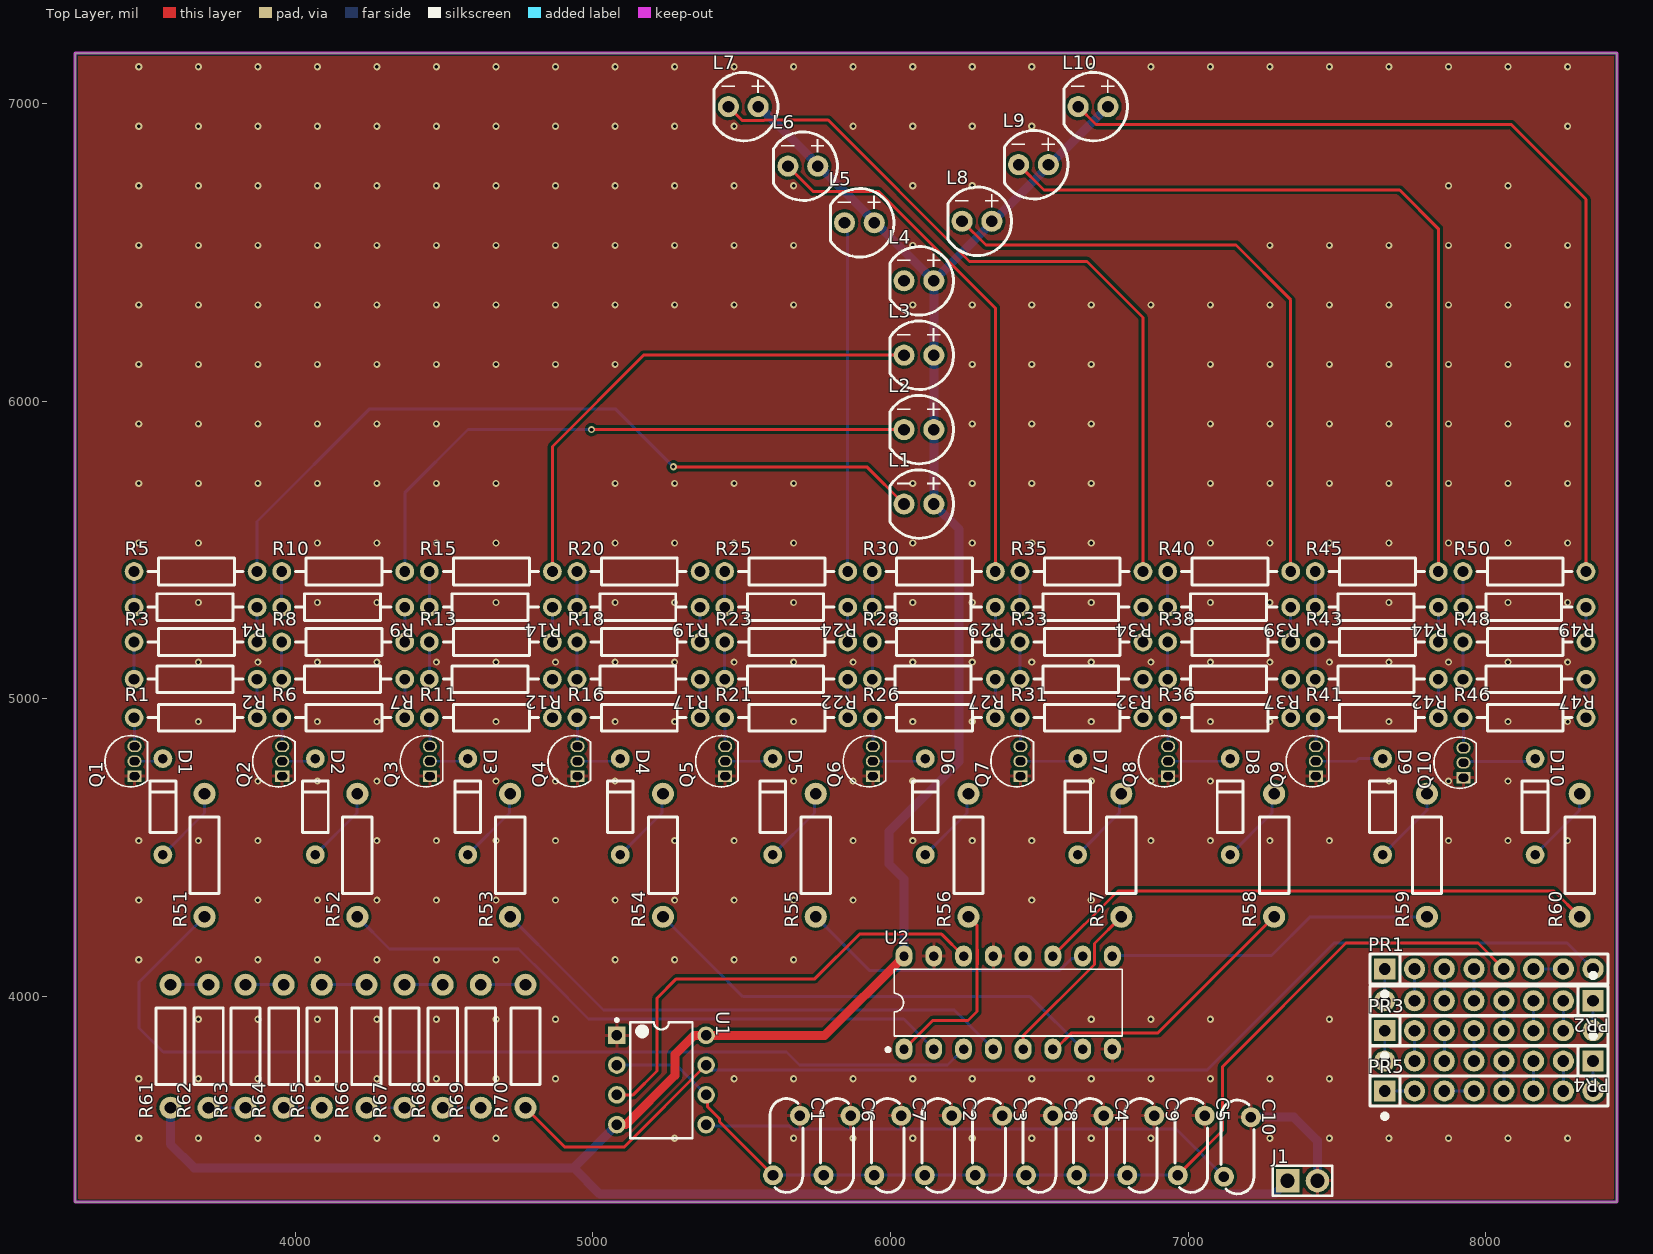
[diagram p0: Top Layer view]
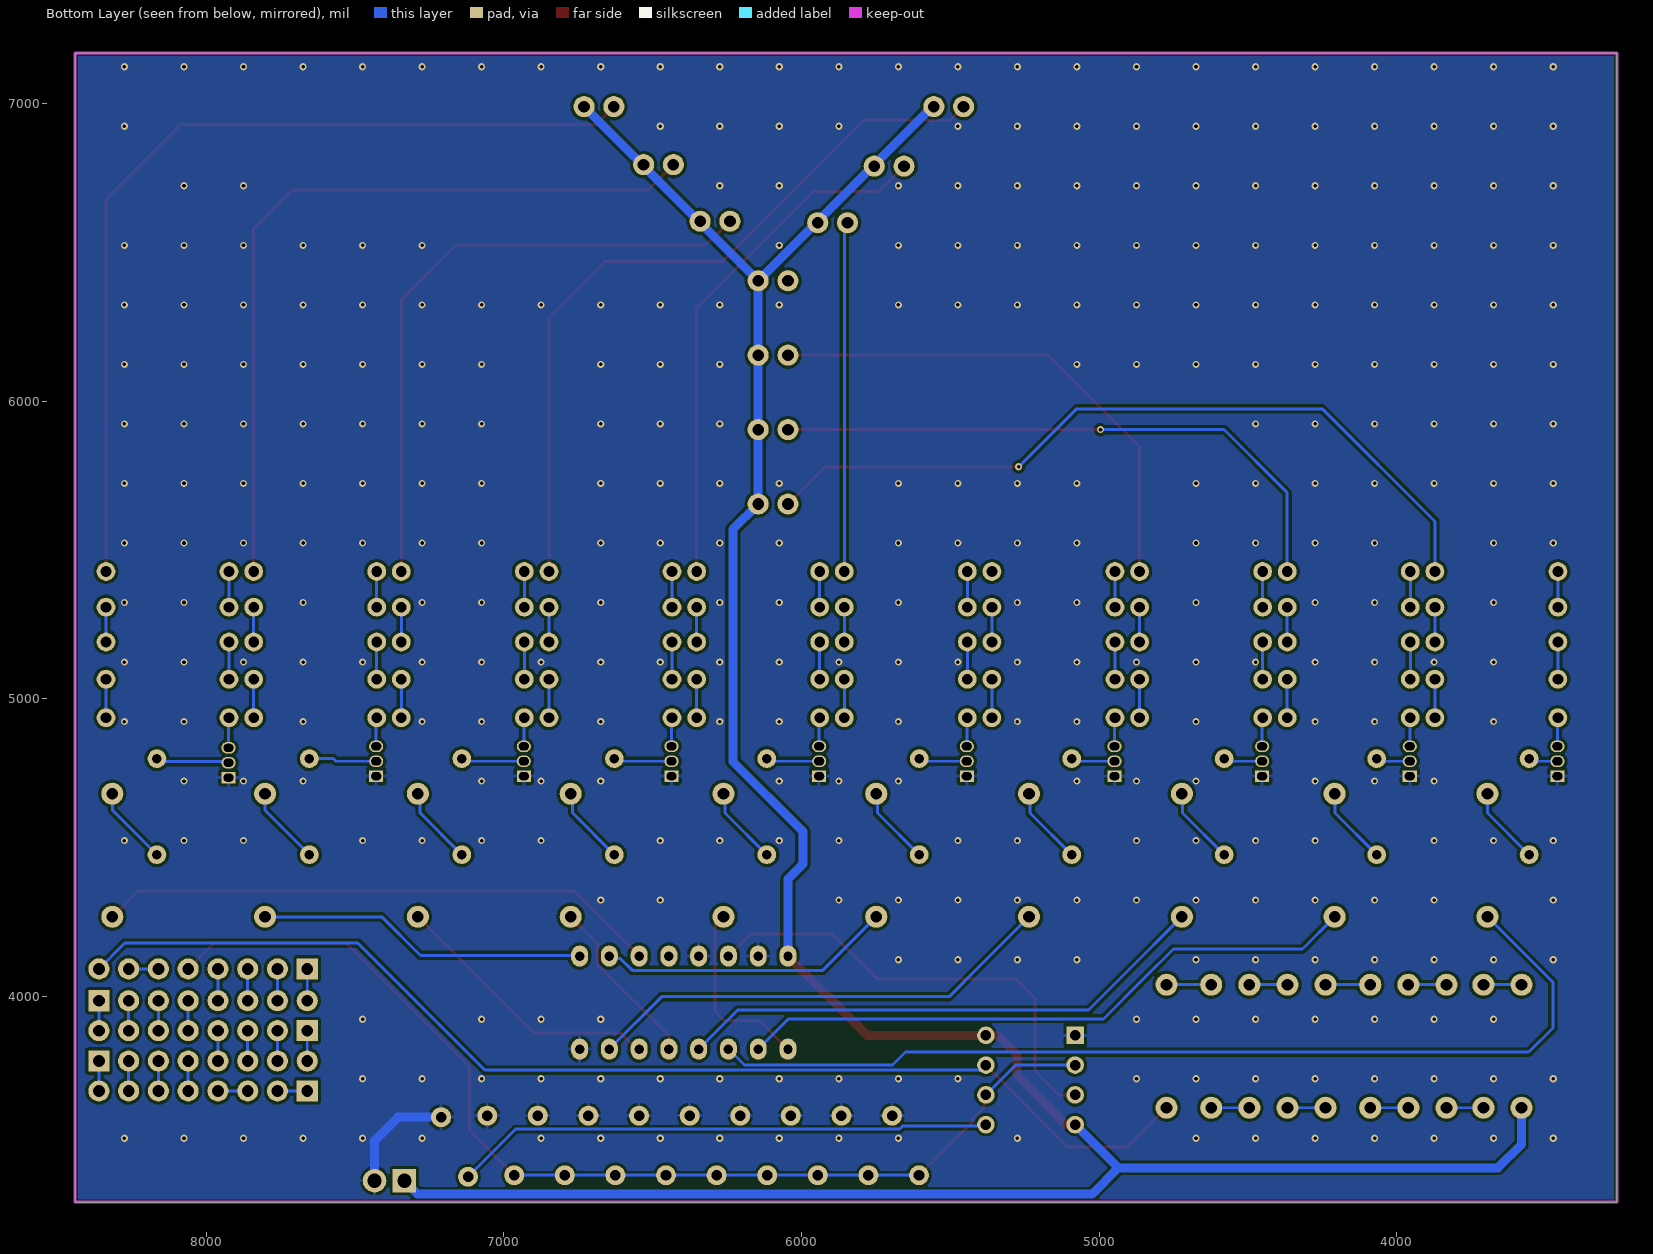
[diagram p1: Bottom Layer view, seen from below]
# Altium PCB MISC51982.pcbdoc
Units mil, origin at the board's own origin, x right, y up, seen from the top; angles counter-clockwise.
Board outline 5180 x 3860 mil, 2 copper layers (Top Layer, Bottom Layer), stack 62.206 mil thick; 118 components, 124 nets, 296 pads, 345 vias.

## Layer stack, top to bottom
Top Solder Mask Layer: solder mask 0.394, Dk 3.3
Top Layer: signal copper 1.379
Dielectric1: surface 59.449, FR4, Dk 4.5
Bottom Layer: signal copper 1.378
Bottom Solder Mask Layer: solder mask 0.394, Dk 3.3

## Board outline
3260,7170 3260,3310 8440,3310 8440,7170

## Design rules (kind name [scope] priority, off if disabled: settings)
BoardOutlineClearance copperThickness2oz_1 [All] p2 off: genericclearance=7.99 ignorepadtopadclearanceinfootprint=FALSE except(0: Arc-SplitContinuation Track-SplitContinuation SMDPad-SplitContinuation THPad-SplitContinuation Via-SplitContinuation Fill-SplitContinuation Region-SplitContinuation Poly-SplitContinuation Text-SplitContinuation Hole-SplitContinuation; 5.98: Arc-CutoutEdge SMDPad-CutoutEdge THPad-CutoutEdge Via-CutoutEdge Fill-CutoutEdge Region-CutoutEdge Text-CutoutEdge; 6.93: Hole-OutlineEdge Hole-CutoutEdge; 10: Poly-OutlineEdge Poly-CutoutEdge; 11.81: Arc-OutlineEdge Track-OutlineEdge SMDPad-OutlineEdge THPad-OutlineEdge Via-OutlineEdge Fill-OutlineEdge Region-OutlineEdge Text-OutlineEdge Track-CutoutEdge)
BoardOutlineClearance Plane_innerPlane_1 [All] p4 off: genericclearance=4.02 ignorepadtopadclearanceinfootprint=FALSE except(0: Arc-SplitContinuation Track-SplitContinuation SMDPad-SplitContinuation THPad-SplitContinuation Via-SplitContinuation Fill-SplitContinuation Region-SplitContinuation Poly-SplitContinuation Text-SplitContinuation Hole-SplitContinuation; 6: SMDPad-CutoutEdge THPad-CutoutEdge Via-CutoutEdge Fill-CutoutEdge Region-CutoutEdge Text-CutoutEdge; 6.93: Hole-OutlineEdge Hole-CutoutEdge; 10: Poly-OutlineEdge Poly-CutoutEdge; 11.8: Arc-OutlineEdge Track-OutlineEdge SMDPad-OutlineEdge THPad-OutlineEdge Via-OutlineEdge Fill-OutlineEdge Region-OutlineEdge Text-OutlineEdge; 11.81: Arc-CutoutEdge Track-CutoutEdge)
BoardOutlineClearance Copper_copperRegion_1 [All] p6 off: genericclearance=4.02 ignorepadtopadclearanceinfootprint=FALSE except(0: Arc-SplitContinuation Track-SplitContinuation SMDPad-SplitContinuation THPad-SplitContinuation Via-SplitContinuation Fill-SplitContinuation Region-SplitContinuation Poly-SplitContinuation Text-SplitContinuation Hole-SplitContinuation; 6: SMDPad-CutoutEdge THPad-CutoutEdge Via-CutoutEdge Fill-CutoutEdge Region-CutoutEdge Text-CutoutEdge; 6.93: Hole-OutlineEdge Hole-CutoutEdge; 10: Poly-OutlineEdge Poly-CutoutEdge; 11.8: Arc-OutlineEdge Track-OutlineEdge SMDPad-OutlineEdge THPad-OutlineEdge Via-OutlineEdge Fill-OutlineEdge Region-OutlineEdge Text-OutlineEdge; 11.81: Arc-CutoutEdge Track-CutoutEdge)
BoardOutlineClearance copperThickness1oz_1 [All] p8: genericclearance=4.02 ignorepadtopadclearanceinfootprint=FALSE except(0: Arc-SplitContinuation Track-SplitContinuation SMDPad-SplitContinuation THPad-SplitContinuation Via-SplitContinuation Fill-SplitContinuation Region-SplitContinuation Poly-SplitContinuation Text-SplitContinuation Hole-SplitContinuation; 6: SMDPad-CutoutEdge THPad-CutoutEdge Via-CutoutEdge Fill-CutoutEdge Region-CutoutEdge Text-CutoutEdge; 6.93: Hole-OutlineEdge Hole-CutoutEdge; 10: Poly-OutlineEdge Poly-CutoutEdge; 11.8: Arc-OutlineEdge Track-OutlineEdge SMDPad-OutlineEdge THPad-OutlineEdge Via-OutlineEdge Fill-OutlineEdge Region-OutlineEdge Text-OutlineEdge; 11.81: Arc-CutoutEdge Track-CutoutEdge)
Clearance copperThickness2oz [All] p1 off: gap=7.99 ignorepadtopadclearanceinfootprint=FALSE except(5.98: SMDPad-Track SMDPad-SMDPad THPad-Track SMDPad-THPad THPad-THPad Track-Via SMDPad-Via THPad-Via Via-Via Fill-Track Region-Track Fill-SMDPad Region-SMDPad Fill-THPad Region-THPad Fill-Via Region-Via Fill-Fill Fill-Region Region-Region Arc-Track Arc-SMDPad Arc-THPad Arc-Via Fill-Arc Region-Arc Arc-Arc Text-Track SMDPad-Text Text-THPad Text-Via Fill-Text Region-Text Arc-Text Text-Text; 6.93: Hole-Track Hole-SMDPad Hole-THPad Hole-Via Fill-Hole Region-Hole Hole-Arc Hole-Text; 10: Poly-Track Poly-SMDPad Poly-THPad Poly-Via Poly-Fill Poly-Region Poly-Poly Poly-Arc Poly-Text Poly-Hole)
Clearance Plane_innerPlane [All] p3 off: gap=4.02 ignorepadtopadclearanceinfootprint=FALSE except(5.98: SMDPad-Track SMDPad-SMDPad THPad-Track SMDPad-THPad THPad-THPad Track-Via SMDPad-Via THPad-Via Via-Via Fill-Track Region-Track Fill-SMDPad Region-SMDPad Fill-THPad Region-THPad Fill-Via Region-Via Fill-Fill Fill-Region Region-Region; 6: Arc-Track Arc-SMDPad Arc-THPad Arc-Via Fill-Arc Region-Arc Arc-Arc Text-Track SMDPad-Text Text-THPad Text-Via Fill-Text Region-Text Arc-Text Text-Text; 6.93: Hole-Track Hole-SMDPad Hole-THPad Hole-Via Fill-Hole Region-Hole Hole-Arc Hole-Text; 10: Poly-Track Poly-SMDPad Poly-THPad Poly-Via Poly-Fill Poly-Region Poly-Poly Poly-Arc Poly-Text Poly-Hole)
Clearance Copper_copperRegion [All] p5 off: gap=4.02 ignorepadtopadclearanceinfootprint=FALSE except(5.98: SMDPad-Track SMDPad-SMDPad THPad-Track SMDPad-THPad THPad-THPad Track-Via SMDPad-Via THPad-Via Via-Via Fill-Track Region-Track Fill-SMDPad Region-SMDPad Fill-THPad Region-THPad Fill-Via Region-Via Fill-Fill Fill-Region Region-Region; 6: Arc-Track Arc-SMDPad Arc-THPad Arc-Via Fill-Arc Region-Arc Arc-Arc Text-Track SMDPad-Text Text-THPad Text-Via Fill-Text Region-Text Arc-Text Text-Text; 6.93: Hole-Track Hole-SMDPad Hole-THPad Hole-Via Fill-Hole Region-Hole Hole-Arc Hole-Text; 10: Poly-Track Poly-SMDPad Poly-THPad Poly-Via Poly-Fill Poly-Region Poly-Poly Poly-Arc Poly-Text Poly-Hole)
Clearance copperThickness1oz [All] p7: gap=4.02 ignorepadtopadclearanceinfootprint=FALSE except(5.98: SMDPad-Track SMDPad-SMDPad THPad-Track SMDPad-THPad THPad-THPad Track-Via SMDPad-Via THPad-Via Via-Via Fill-Track Region-Track Fill-SMDPad Region-SMDPad Fill-THPad Region-THPad Fill-Via Region-Via Fill-Fill Fill-Region Region-Region; 6: Arc-Track Arc-SMDPad Arc-THPad Arc-Via Fill-Arc Region-Arc Arc-Arc Text-Track SMDPad-Text Text-THPad Text-Via Fill-Text Region-Text Arc-Text Text-Text; 6.93: Hole-Track Hole-SMDPad Hole-THPad Hole-Via Fill-Hole Region-Hole Hole-Arc Hole-Text; 10: Poly-Track Poly-SMDPad Poly-THPad Poly-Via Poly-Fill Poly-Region Poly-Poly Poly-Arc Poly-Text Poly-Hole)
DiffPairsRouting differentialPair [All] p1: maxlimit=6 minlimit=6 mostfreqgap=6 toplayer_minwidth=5 toplayer_prefwidth=10 toplayer_maxwidth=100 toplayer_mingap=6 toplayer_prefgap=6 toplayer_maxgap=6 bottomlayer_minwidth=5 bottomlayer_prefwidth=10 bottomlayer_maxwidth=100 bottomlayer_mingap=6 bottomlayer_prefgap=6 bottomlayer_maxgap=6 maxuncoupledlength=10
HoleToHoleClearance otherClearance [All] p1: gap=11.81 allowstackedmicrovias=TRUE
Length netLength [All] p1: minlimit=0 maxlimit=0
PasteMaskExpansion pasteMaskExpansion [All] p1: expansion=0
PlaneConnect innerPlane [All] p1: planeconnectstyle=Relief reliefexpansion=20 reliefentries=4 reliefconductorwidth=10 reliefairgap=10
PolygonConnect copperRegion [All] p1: connectstyle=Relief reliefconductorwidth=10 reliefentries=4 polygonreliefangle="90 Angle" airgapwidth=10 via.connectstyle=Relief via.reliefconductorwidth=10 via.reliefentries=4 via.polygonreliefangle="90 Angle" via.airgapwidth=10
RoutingVias viaSize [All] p1: holewidth=12.01 width=24.02 viastyle="Through Hole" minholewidth=11.81 minwidth=19.68 maxholewidth=248.03 maxwidth=393.7
SolderMaskExpansion solderMaskExpansion [IsVia] p1: expansion=-1000 istentingtop=TRUE
SolderMaskExpansion solderMaskExpansion [All] p2: expansion=2 istentingtop=FALSE
Width copperThickness2oz_2 [All] p1 off: maxlimit=100 minlimit=8 preferedwidth=10
Width copperThickness1oz_2 [All] p2: maxlimit=100 minlimit=5 preferedwidth=10

## Components (designator, comment, footprint, x,y, rotation, side; value= is the part's Value field where it differs from the comment)
C1 "10nF" CAP-TH_L8.0-W2.8-P5.08-D0.6 5650,3500 r270 top
C2 "10nF" CAP-TH_L8.0-W2.8-P5.08-D0.6 6160,3500 r270 top
C3 "10nF" CAP-TH_L8.0-W2.8-P5.08-D0.6 6330,3500 r270 top
C4 "10nF" CAP-TH_L8.0-W2.8-P5.08-D0.6 6670,3500 r270 top
C5 "10nF" CAP-TH_L8.0-W2.8-P5.08-D0.6 7010,3500 r270 top
C6 "10nF" CAP-TH_L8.0-W2.8-P5.08-D0.6 5820,3500 r270 top
C7 "10nF" CAP-TH_L8.0-W2.8-P5.08-D0.6 5990,3500 r270 top
C8 "10nF" CAP-TH_L8.0-W2.8-P5.08-D0.6 6500,3500 r270 top
C9 "10nF" CAP-TH_L8.0-W2.8-P5.08-D0.6 6840,3500 r270 top
C10 "10nF" CAP-TH_L8.0-W2.8-P5.08-D0.6 7165,3495 r270 top
D1 "1N4148TR" DO-35_BD2.0-L4.2-P8.20-D0.5-RD 3555,4638.39 r270 top
D2 "1N4148TR" DO-35_BD2.0-L4.2-P8.20-D0.5-RD 4067.22,4638.39 r270 top
D3 "1N4148TR" DO-35_BD2.0-L4.2-P8.20-D0.5-RD 4579.44,4638.39 r270 top
D4 "1N4148TR" DO-35_BD2.0-L4.2-P8.20-D0.5-RD 5091.67,4638.39 r270 top
D5 "1N4148TR" DO-35_BD2.0-L4.2-P8.20-D0.5-RD 5603.89,4638.39 r270 top
D6 "1N4148TR" DO-35_BD2.0-L4.2-P8.20-D0.5-RD 6116.11,4638.39 r270 top
D7 "1N4148TR" DO-35_BD2.0-L4.2-P8.20-D0.5-RD 6628.33,4638.39 r270 top
D8 "1N4148TR" DO-35_BD2.0-L4.2-P8.20-D0.5-RD 7140.56,4638.39 r270 top
D9 "1N4148TR" DO-35_BD2.0-L4.2-P8.20-D0.5-RD 7652.78,4638.39 r270 top
D10 "1N4148TR" DO-35_BD2.0-L4.2-P8.20-D0.5-RD 8165,4638.39 r270 top
J1 "PZ254V-11-02P" HDR-TH_2P-P2.54-V-M 7383.93,3381.56 r0 top
L1 "XL-502SURD" LED-TH_BD5.9-P2.54-RD_RED 6095,5655 r0 top
L2 "XL-502SURD" LED-TH_BD5.9-P2.54-RD_RED 6095,5905 r0 top
L3 "XL-502SURD" LED-TH_BD5.9-P2.54-RD_RED 6095,6155 r0 top
L4 "XL-502SURD" LED-TH_BD5.9-P2.54-RD_RED 6095,6405 r0 top
L5 "XL-502SURD" LED-TH_BD5.9-P2.54-RD_RED 5895,6600 r0 top
L6 "XL-502SURD" LED-TH_BD5.9-P2.54-RD_RED 5705,6790 r0 top
L7 "XL-502SURD" LED-TH_BD5.9-P2.54-RD_RED 5505,6990 r0 top
L8 "XL-502SURD" LED-TH_BD5.9-P2.54-RD_RED 6290,6605 r0 top
L9 "XL-502SURD" LED-TH_BD5.9-P2.54-RD_RED 6480,6795 r0 top
L10 "XL-502SURD" LED-TH_BD5.9-P2.54-RD_RED 6680,6990 r0 top
PR1 "10kΩ" RES-ARRAY-TH_8P-L20.3-W2.5-P2.54 8010,4093.09 r0 top
PR2 "10kΩ" RES-ARRAY-TH_8P-L20.3-W2.5-P2.54 8010,3986.11 r180 top
PR3 "10kΩ" RES-ARRAY-TH_8P-L20.3-W2.5-P2.54 8010,3885.62 r0 top
PR4 "10kΩ" RES-ARRAY-TH_8P-L20.3-W2.5-P2.54 8010,3783.65 r180 top
PR5 "10kΩ" RES-ARRAY-TH_8P-L20.3-W2.5-P2.54 8010,3683.16 r0 top
Q1 "S8050" TO-92-3_L4.5-W3.5-P1.27-L 3459.84,4790.8 r90 top
Q2 "S8050" TO-92-3_L4.5-W3.5-P1.27-L 3955.91,4790.8 r90 top
Q3 "S8050" TO-92-3_L4.5-W3.5-P1.27-L 4451.98,4790.8 r90 top
Q4 "S8050" TO-92-3_L4.5-W3.5-P1.27-L 4948.05,4790.8 r90 top
Q5 "S8050" TO-92-3_L4.5-W3.5-P1.27-L 5444.11,4790.8 r90 top
Q6 "S8050" TO-92-3_L4.5-W3.5-P1.27-L 5940.18,4790.8 r90 top
Q7 "S8050" TO-92-3_L4.5-W3.5-P1.27-L 6436.25,4790.8 r90 top
Q8 "S8050" TO-92-3_L4.5-W3.5-P1.27-L 6932.31,4790.8 r90 top
Q9 "S8050" TO-92-3_L4.5-W3.5-P1.27-L 7428.38,4790.8 r90 top
Q10 "S8050" TO-92-3_L4.5-W3.5-P1.27-L 7924.45,4785.8 r90 top
R1 "100Ω" RES-TH_BD2.2-L6.5-P10.50-D0.6 3664.84,4937.09 r0 top
R2 "100Ω" RES-TH_BD2.2-L6.5-P10.50-D0.6 3664.84,5066.43 r180 top
R3 "100Ω" RES-TH_BD2.2-L6.5-P10.50-D0.6 3664.84,5191.55 r0 top
R4 "100Ω" RES-TH_BD2.2-L6.5-P10.50-D0.6 3664.84,5308.56 r180 top
R5 "100Ω" RES-TH_BD2.2-L6.5-P10.50-D0.6 3664.84,5428.24 r0 top
R6 "100Ω" RES-TH_BD2.2-L6.5-P10.50-D0.6 4160.91,4937.09 r0 top
R7 "100Ω" RES-TH_BD2.2-L6.5-P10.50-D0.6 4160.91,5066.43 r180 top
R8 "100Ω" RES-TH_BD2.2-L6.5-P10.50-D0.6 4160.91,5191.55 r0 top
R9 "100Ω" RES-TH_BD2.2-L6.5-P10.50-D0.6 4160.91,5308.56 r180 top
R10 "100Ω" RES-TH_BD2.2-L6.5-P10.50-D0.6 4160.91,5428.24 r0 top
R11 "100Ω" RES-TH_BD2.2-L6.5-P10.50-D0.6 4656.98,4937.09 r0 top
R12 "100Ω" RES-TH_BD2.2-L6.5-P10.50-D0.6 4656.98,5066.43 r180 top
R13 "100Ω" RES-TH_BD2.2-L6.5-P10.50-D0.6 4656.98,5191.55 r0 top
R14 "100Ω" RES-TH_BD2.2-L6.5-P10.50-D0.6 4656.98,5308.56 r180 top
R15 "100Ω" RES-TH_BD2.2-L6.5-P10.50-D0.6 4656.98,5428.24 r0 top
R16 "100Ω" RES-TH_BD2.2-L6.5-P10.50-D0.6 5153.05,4937.09 r0 top
R17 "100Ω" RES-TH_BD2.2-L6.5-P10.50-D0.6 5153.05,5066.43 r180 top
R18 "100Ω" RES-TH_BD2.2-L6.5-P10.50-D0.6 5153.05,5191.55 r0 top
R19 "100Ω" RES-TH_BD2.2-L6.5-P10.50-D0.6 5153.05,5308.56 r180 top
R20 "100Ω" RES-TH_BD2.2-L6.5-P10.50-D0.6 5153.05,5428.24 r0 top
R21 "100Ω" RES-TH_BD2.2-L6.5-P10.50-D0.6 5649.11,4937.09 r0 top
R22 "100Ω" RES-TH_BD2.2-L6.5-P10.50-D0.6 5649.11,5066.43 r180 top
R23 "100Ω" RES-TH_BD2.2-L6.5-P10.50-D0.6 5649.11,5191.55 r0 top
R24 "100Ω" RES-TH_BD2.2-L6.5-P10.50-D0.6 5649.11,5308.56 r180 top
R25 "100Ω" RES-TH_BD2.2-L6.5-P10.50-D0.6 5649.11,5428.24 r0 top
R26 "100Ω" RES-TH_BD2.2-L6.5-P10.50-D0.6 6145.18,4937.09 r0 top
R27 "100Ω" RES-TH_BD2.2-L6.5-P10.50-D0.6 6145.18,5066.43 r180 top
R28 "100Ω" RES-TH_BD2.2-L6.5-P10.50-D0.6 6145.18,5191.55 r0 top
R29 "100Ω" RES-TH_BD2.2-L6.5-P10.50-D0.6 6145.18,5308.56 r180 top
R30 "100Ω" RES-TH_BD2.2-L6.5-P10.50-D0.6 6145.18,5428.24 r0 top
R31 "100Ω" RES-TH_BD2.2-L6.5-P10.50-D0.6 6641.25,4937.09 r0 top
R32 "100Ω" RES-TH_BD2.2-L6.5-P10.50-D0.6 6641.25,5066.43 r180 top
R33 "100Ω" RES-TH_BD2.2-L6.5-P10.50-D0.6 6641.25,5191.55 r0 top
R34 "100Ω" RES-TH_BD2.2-L6.5-P10.50-D0.6 6641.25,5308.56 r180 top
R35 "100Ω" RES-TH_BD2.2-L6.5-P10.50-D0.6 6641.25,5428.24 r0 top
R36 "100Ω" RES-TH_BD2.2-L6.5-P10.50-D0.6 7137.31,4937.09 r0 top
R37 "100Ω" RES-TH_BD2.2-L6.5-P10.50-D0.6 7137.31,5066.43 r180 top
R38 "100Ω" RES-TH_BD2.2-L6.5-P10.50-D0.6 7137.31,5191.55 r0 top
R39 "100Ω" RES-TH_BD2.2-L6.5-P10.50-D0.6 7137.31,5308.56 r180 top
R40 "100Ω" RES-TH_BD2.2-L6.5-P10.50-D0.6 7137.31,5428.24 r0 top
R41 "100Ω" RES-TH_BD2.2-L6.5-P10.50-D0.6 7633.38,4937.09 r0 top
R42 "100Ω" RES-TH_BD2.2-L6.5-P10.50-D0.6 7633.38,5066.43 r180 top
R43 "100Ω" RES-TH_BD2.2-L6.5-P10.50-D0.6 7633.38,5191.55 r0 top
R44 "100Ω" RES-TH_BD2.2-L6.5-P10.50-D0.6 7633.38,5308.56 r180 top
R45 "100Ω" RES-TH_BD2.2-L6.5-P10.50-D0.6 7633.38,5428.24 r0 top
R46 "100Ω" RES-TH_BD2.2-L6.5-P10.50-D0.6 8129.45,4937.09 r0 top
R47 "100Ω" RES-TH_BD2.2-L6.5-P10.50-D0.6 8129.45,5066.43 r180 top
R48 "100Ω" RES-TH_BD2.2-L6.5-P10.50-D0.6 8129.45,5191.55 r0 top
R49 "100Ω" RES-TH_BD2.2-L6.5-P10.50-D0.6 8129.45,5308.56 r180 top
R50 "100Ω" RES-TH_BD2.2-L6.5-P10.50-D0.6 8129.45,5428.24 r0 top
R51 "1kΩ" RES-TH_BD2.5-L6.5-P10.50-D0.6 3695,4475 r90 top
R52 "1kΩ" RES-TH_BD2.5-L6.5-P10.50-D0.6 4208.33,4475 r90 top
R53 "1kΩ" RES-TH_BD2.5-L6.5-P10.50-D0.6 4721.67,4475 r90 top
R54 "1kΩ" RES-TH_BD2.5-L6.5-P10.50-D0.6 5235,4475 r90 top
R55 "1kΩ" RES-TH_BD2.5-L6.5-P10.50-D0.6 5748.33,4475 r90 top
R56 "1kΩ" RES-TH_BD2.5-L6.5-P10.50-D0.6 6261.67,4475 r90 top
R57 "1kΩ" RES-TH_BD2.5-L6.5-P10.50-D0.6 6775,4475 r90 top
R58 "1kΩ" RES-TH_BD2.5-L6.5-P10.50-D0.6 7288.33,4475 r90 top
R59 "1kΩ" RES-TH_BD2.5-L6.5-P10.50-D0.6 7801.67,4475 r90 top
R60 "1kΩ" RES-TH_BD2.5-L6.5-P10.50-D0.6 8315,4475 r90 top
R61 "1kΩ" RES-TH_BD2.5-L6.5-P10.50-D0.6 3580.49,3833.38 r90 top
R62 "1kΩ" RES-TH_BD2.5-L6.5-P10.50-D0.6 3708.6,3833.38 r90 top
R63 "1kΩ" RES-TH_BD2.5-L6.5-P10.50-D0.6 3832.5,3833.38 r90 top
R64 "1kΩ" RES-TH_BD2.5-L6.5-P10.50-D0.6 3960.61,3833.38 r90 top
R65 "1kΩ" RES-TH_BD2.5-L6.5-P10.50-D0.6 4088.72,3833.38 r90 top
R66 "1kΩ" RES-TH_BD2.5-L6.5-P10.50-D0.6 4238.72,3833.38 r90 top
R67 "1kΩ" RES-TH_BD2.5-L6.5-P10.50-D0.6 4366.83,3833.38 r90 top
R68 "1kΩ" RES-TH_BD2.5-L6.5-P10.50-D0.6 4494.94,3833.38 r90 top
R69 "1kΩ" RES-TH_BD2.5-L6.5-P10.50-D0.6 4623.05,3833.38 r90 top
R70 "1kΩ" RES-TH_BD2.5-L6.5-P10.50-D0.6 4773.05,3833.38 r90 top
U1 "NE555P" DIP-8_L9.8-W6.6-P2.54-LS7.6-BL 5230,3720 r270 top
U2 "CD4017CN" PDIP-16_L19.3-W6.4-P2.54-LS7.94-BL 6395,3980 r0 top

## Footprints (in the part's own frame and the unit in brackets; to place one, negate y for a bottom-side part, rotate by r counter-clockwise, add the part's x,y. Pads: shape width x height; smd on the part's side, far side on the other; paste and mask are expansions set on the pad)
CAP-TH_L8.0-W2.8-P5.08-D0.6 [mm]
  round 1.7 hole 0.9 paste+0 mask+0.05: 1(-2.54,1.15) 2(2.54,-1.15)
  silkscreen extent -4,-1.4 4,1.4
DIP-8_L9.8-W6.6-P2.54-LS7.6-BL [mm]
  rect 1.5x1.5 hole 0.9: 1(-3.81,-3.81)
  round 1.5 hole 0.9: 2(-1.27,-3.81) 3(1.27,-3.81) 4(3.81,-3.81) 5(3.81,3.81) 6(1.27,3.81) 7(-1.27,3.81) 8(-3.81,3.81)
  silkscreen extent -5.23,-3.93 4.96,2.65
DO-35_BD2.0-L4.2-P8.20-D0.5-RD [mm]
  round 1.6 hole 0.8: 1(-4.1,0) 2(4.1,0)
  silkscreen extent -2.2,-1.1 2.2,1.1
HDR-TH_2P-P2.54-V-M [mm]
  rect 2x2 hole 1.2: 1(-1.27,0)
  round 2 hole 1.2: 2(1.27,0)
  silkscreen extent -2.54,-1.27 2.54,1.27
LED-TH_BD5.9-P2.54-RD_RED [mm]
  round 1.8 hole 1 paste+0 mask+0.05: 1(-1.27,0) 2(1.27,0)
  silkscreen extent -2.49,-2.92 2.94,2.92
PDIP-16_L19.3-W6.4-P2.54-LS7.94-BL [mm]
  oval 1.44x1.8 hole 0.8: 1(-8.89,-3.97) 2(-6.35,-3.97) 3(-3.81,-3.97) 4(-1.27,-3.97) 5(1.27,-3.97) 6(3.81,-3.97) 7(6.35,-3.97) 8(8.89,-3.97) 9(8.89,3.97) 10(6.35,3.97) 11(3.81,3.97) 12(1.27,3.97) 13(-1.27,3.97) 14(-3.81,3.97) 15(-6.35,3.97) 16(-8.89,3.97)
  silkscreen extent -10.41,-4.17 9.73,2.84
RES-ARRAY-TH_8P-L20.3-W2.5-P2.54 [mm]
  rect 1.8x1.8 hole 1: 1(-8.89,0)
  round 1.8 hole 1: 2(-6.35,0) 3(-3.81,0) 4(-1.27,0) 5(1.27,0) 6(3.81,0) 7(6.35,0) 8(8.89,0)
  silkscreen extent -10.16,-2.36 10.16,1.27
RES-TH_BD2.2-L6.5-P10.50-D0.6 [mm]
  round 1.6 hole 0.914: 1(-5.25,0) 2(5.25,0)
  silkscreen extent -4.06,-1.14 4.06,1.14
RES-TH_BD2.5-L6.5-P10.50-D0.6 [mil]
  round 74 hole 39.37: 1(-206.69,0) 2(206.69,0)
  silkscreen extent -128,-49 128,49
TO-92-3_L4.5-W3.5-P1.27-L [mm]
  rect 1x1.2 hole 0.7 slot 0.85 at 90 deg: 1(-1.27,0)
  oval 1x1.2 hole 0.7 slot 0.85 at 90 deg: 2(0,0) 3(1.27,0)
  silkscreen extent -2.19,-1.1 2.19,2.52

## Via types
v1: diameter 24.02, hole 12, Top Layer to Bottom Layer, 345 vias

## Nets (pads, with @x,y where several pads share a name; then routed paths per layer and width w, separated by ;. In a path a pad name is that pad's centre, name@x,y a point inside that pad or via, vN(x,y) a via of type N, cw(c..) or ccw(c..) an arc to the next point about the centre after c; other vN are vias at no path point)
$1N509: U1.3 U2.14 | length 1562.7
  Top Layer w10: U1.3 5135,3670 5215,3750 5215,3995 5280,4060 5745,4060 5895,4210 6171.3,4210 U2.14
$1N552: C10.2 U1.5 | length 1811.3
  Bottom Layer w10: U1.5 5389.72,3565 5659.72,3565 5669.72,3555 6959.72,3555 C10.2
$1N1039: R60.1 U2.11 | length 1896.5
  Top Layer w10: U2.11 6763.7,4355 8228.31,4355 R60.1
$1N1041: R59.1 U2.9 | length 1110.6
  Bottom Layer w10: U2.9 6761.67,4138.31 7279.71,4138.31 7409.71,4268.31 R59.1
$1N1043: R58.1 U2.6 | length 927.5
  Top Layer w10: U2.6 6553.73,3823.7 6608.34,3878.31 6898.34,3878.31 R58.1
$1N1045: R57.1 U2.5 | length 581.3
  Top Layer w10: U2.5 6445,3868.31 6685,4108.31 6685,4178.31 R57.1
$1N1047: R56.1 U2.1 | length 692.2
  Top Layer w10: R56.1 6290,4239.98 6290,4159.98 ; U2.1@6051.67,3830.37 6051.67,3828.31 U2.1 U2.1@6051.67,3830.37 ; U2.1@6051.67,3830.37 6141.3,3920 6260,3920 6290,3950 6290,4106.64 ; 6290,4106.64 6290,4159.98 ; 6290,4106.64 6291.67,4108.31 6291.67,4158.31 6290,4159.98
$1N1049: R55.1 U2.10 | length 989.6
  Bottom Layer w10: R55.1 5928.33,4088.31 6568.33,4088.31 6608.33,4128.31 6628.33,4128.31 U2.10
$1N1051: R54.1 U2.7 | length 1594.2
  Bottom Layer w10: R54.1 5402.89,4100.42 5503.31,4000 6468.7,4000 U2.7
$1N1053: R53.1 U2.4 | length 1807.5
  Bottom Layer w10: R53.1 4912.26,4077.72 5034.98,3955 6213.7,3955 U2.4
$1N1055: R51.1 U2.3 | length 3308.5
  Bottom Layer w10: R51.1 3475,4048.31 3475,3895 3556.3,3813.7 5650.32,3813.7 5694.02,3770 6191.3,3770 U2.3
$1N1057: R52.1 U2.2 | length 2120.8
  Bottom Layer w10: R52.1 4316.64,4160 4750,4160 4847.69,4062.31 4985,3925 6043.7,3925 U2.2
$1N1689: R4.2 R5.1 | length 119.7
  Bottom Layer w10: R4.2@3458.15,5308.56 R5.1
$1N1693: R3.2 R4.1 | length 117
  Bottom Layer w10: R3.2 R4.1
$1N1698: R2.2 R3.1 | length 125.1
  Bottom Layer w10: R2.2@3458.15,5066.43 R3.1
$1N1703: R1.2 R2.1 | length 129.3
  Bottom Layer w10: R1.2 R2.1
$1N1886: R6.2 R7.1 | length 129.3
  Bottom Layer w10: R6.2 R7.1
$1N1888: R8.2 R9.1 | length 117
  Bottom Layer w10: R8.2 R9.1
$1N1890: R7.2 R8.1 | length 125.1
  Bottom Layer w10: R7.2 R8.1
$1N1892: R9.2 R10.1 | length 119.7
  Bottom Layer w10: R9.2 R10.1
$1N2074: R11.2 R12.1 | length 129.3
  Bottom Layer w10: R11.2 R12.1
$1N2076: R13.2 R14.1 | length 117
  Bottom Layer w10: R13.2 R14.1
$1N2078: R12.2 R13.1 | length 125.1
  Bottom Layer w10: R12.2 R13.1
$1N2080: R14.2 R15.1 | length 119.7
  Bottom Layer w10: R14.2 R15.1
$1N2826: R16.2 R17.1 | length 129.3
  Bottom Layer w10: R16.2 R17.1
$1N2828: R18.2 R19.1 | length 117
  Bottom Layer w10: R18.2 R19.1
$1N2830: R17.2 R18.1 | length 125.1
  Bottom Layer w10: R17.2@4946.35,5066.43 R18.1@4946.35,5191.54
$1N2832: R19.2 R20.1 | length 119.7
  Bottom Layer w10: R19.2@4946.35,5308.56 R20.1@4946.35,5428.24
$1N3014: R21.2 R22.1 | length 129.3
  Bottom Layer w10: R21.2 R22.1
$1N3016: R23.2 R24.1 | length 117
  Bottom Layer w10: R23.2 R24.1
$1N3018: R22.2 R23.1 | length 125.1
  Bottom Layer w10: R22.2 R23.1
$1N3020: R24.2 R25.1 | length 119.7
  Bottom Layer w10: R24.2 R25.1
$1N4862: R32.2 R33.1 | length 125.1
  Bottom Layer w10: R32.2@6434.55,5066.43 R33.1@6434.55,5191.54
$1N4864: R33.2 R34.1 | length 117
  Bottom Layer w10: R33.2 R34.1
$1N4866: R31.2 R32.1 | length 129.3
  Bottom Layer w10: R31.2 R32.1
$1N4868: R34.2 R35.1 | length 119.7
  Bottom Layer w10: R34.2@6434.55,5308.56 R35.1@6434.55,5428.24
$1N4870: R26.2 R27.1 | length 129.3
  Bottom Layer w10: R26.2 R27.1
$1N4872: R27.2 R28.1 | length 125.1
  Bottom Layer w10: R27.2 R28.1
$1N4874: R28.2 R29.1 | length 117
  Bottom Layer w10: R28.2 R29.1
$1N4876: R29.2 R30.1 | length 119.7
  Bottom Layer w10: R29.2 R30.1
$1N4878: R37.2 R38.1 | length 125.1
  Bottom Layer w10: R37.2 R38.1
$1N4880: R39.2 R40.1 | length 119.7
  Bottom Layer w10: R39.2 R40.1
$1N4882: R36.2 R37.1 | length 129.3
  Bottom Layer w10: R36.2 R37.1
$1N4884: R38.2 R39.1 | length 117
  Bottom Layer w10: R38.2 R39.1
$1N4886: R47.2 R48.1 | length 125.1
  Bottom Layer w10: R47.2 R48.1
$1N4888: R48.2 R49.1 | length 117
  Bottom Layer w10: R48.2 R49.1
$1N4890: R46.2 R47.1 | length 129.3
  Bottom Layer w10: R46.2 R47.1
$1N4892: R49.2 R50.1 | length 119.7
  Bottom Layer w10: R49.2 R50.1
$1N4894: R44.2 R45.1 | length 119.7
  Bottom Layer w10: R44.2 R45.1
$1N4896: R43.2 R44.1 | length 117
  Bottom Layer w10: R43.2 R44.1
$1N4898: R42.2 R43.1 | length 125.1
  Bottom Layer w10: R42.2 R43.1
$1N4900: R41.2 R42.1 | length 129.3
  Bottom Layer w10: R41.2 R42.1
$1N6278: D1.2 R51.2 | length 262.7
  Bottom Layer w10: D1.2 3695,4616.97 R51.2
$1N6282: D2.2 R52.2 | length 262.8
  Bottom Layer w10: D2.2 4207.22,4616.97 4207.22,4666.97 R52.2
$1N6287: D3.2 R53.2 | length 262.9
  Bottom Layer w10: D3.2 4719.44,4616.97 4719.44,4666.97 R53.2
$1N6292: D4.2 R54.2 | length 263.1
  Bottom Layer w10: D4.2 5231.67,4616.97 5231.67,4666.97 R54.2
$1N6297: D5.2 R55.2 | length 263.4
  Bottom Layer w10: D5.2 5743.89,4616.97 5743.89,4666.97 R55.2
$1N6302: D6.2 R56.2 | length 263.7
  Bottom Layer w10: D6.2 6256.11,4616.97 6256.11,4666.97 R56.2
$1N6307: D7.2 R57.2 | length 264.2
  Bottom Layer w10: D7.2 6768.33,4616.97 6768.33,4666.97 R57.2
$1N6312: D8.2 R58.2 | length 264.6
  Bottom Layer w10: D8.2 7280.56,4616.97 7280.56,4666.97 R58.2
$1N6317: D9.2 R59.2 | length 266.4
  Bottom Layer w10: D9.2 7801.67,4625.86 R59.2
$1N6322: D10.2 R60.2 | length 266.9
  Bottom Layer w10: D10.2 8315,4626.97 R60.2
$1N6789: Q10.3 R46.1 | length 102
  Bottom Layer w10: R46.1 7924.45,4935.4 Q10.3
$1N6799: Q9.3 R41.1 | length 97
  Bottom Layer w10: R41.1 7426.69,4932.5 7428.38,4930.8 Q9.3
$1N6801: Q8.3 R36.1 | length 96.5
  Bottom Layer w10: R36.1 6932.31,4930.8 Q8.3
$1N6803: Q7.3 R31.1 | length 96.5
  Bottom Layer w10: R31.1@6434.55,4937.09 6436.25,4930.8 Q7.3
$1N6805: Q6.3 R26.1 | length 96.5
  Bottom Layer w10: R26.1 5940.18,4930.8 Q6.3
$1N6807: Q5.3 R21.1 | length 96.5
  Bottom Layer w10: R21.1 5444.11,4930.8 Q5.3
$1N6809: Q4.3 R16.1 | length 96.5
  Bottom Layer w10: R16.1@4946.35,4937.09 4948.04,4930.8 Q4.3
$1N6811: Q3.3 R11.1 | length 97
  Bottom Layer w10: R11.1 4450.28,4932.5 4451.98,4930.8 Q3.3
$1N6813: Q2.3 R6.1 | length 96.5
  Bottom Layer w10: R6.1 3955.91,4930.8 Q2.3
$1N6815: Q1.3 R1.1 | length 96.5
  Bottom Layer w10: R1.1 3459.84,4930.8 Q1.3
$1N6819: D1.1 Q1.2 | length 98.9
  Bottom Layer w10: Q1.2 3525.99,4790.8 3535,4799.81 D1.1
$1N6827: D2.1 Q2.2 | length 115
  Bottom Layer w10: Q2.2 4038.22,4790.8 4047.22,4799.81 D2.1
$1N6833: D3.1 Q3.2 | length 131.2
  Bottom Layer w10: Q3.2 4560.43,4790.8 4569.44,4799.81 D3.1
$1N6840: D4.1 Q4.2 | length 147.4
  Bottom Layer w10: Q4.2 5072.66,4790.8 5081.67,4799.81 D4.1
$1N6847: D5.1 Q5.2 | length 163.5
  Bottom Layer w10: Q5.2 5584.88,4790.8 5593.89,4799.81 D5.1
$1N6854: D6.1 Q6.2 | length 179.7
  Bottom Layer w10: Q6.2 6107.1,4790.8 D6.1
$1N6860: D7.1 Q7.2 | length 195.8
  Bottom Layer w10: Q7.2 6619.32,4790.8 D7.1
$1N6867: D8.1 Q8.2 | length 212
  Bottom Layer w10: Q8.2 7131.55,4790.8 D8.1
$1N6874: D9.1 Q9.2 | length 228.1
  Bottom Layer w10: Q9.2 7563.77,4790.8 7572.78,4799.81 D9.1
$1N6881: D10.1 Q10.2 | length 245.4
  Bottom Layer w10: Q10.2 7935,4789.81 8155,4789.81 D10.1
$1N7123: L1.1 R5.2 | length 2631.1
  Top Layer w10: v1(5270,5780) 5920,5780 L1.1
  Bottom Layer w10: R5.2 3871.54,5596.54 4250,5975 5075,5975 v1(5270,5780)
$1N7169: L2.1 R10.2 | length 2052.3
  Top Layer w10: v1(4995,5905) L2.1
  Bottom Layer w10: R10.2@4390,5430 4380,5430 R10.2 4367.61,5692.61 4580,5905 v1(4995,5905)
$1N7259: L3.1 R15.2 | length 1746.9
  Top Layer w10: R15.2 4863.67,5848.67 5170,6155 L3.1
  Bottom Layer w10: R15.2 4871.98,5428.08 R15.2@4881.98,5428.08
$1N7261: L4.1
$1N7351: L5.1 R25.2 | length 1176.2
  Bottom Layer w10: L5.1 5855.81,6589.19 R25.2
$1N7353: L6.1 R30.2 | length 1779.3
  Top Layer w10: L6.1 5740,6705 5960,6705 6351.87,6313.13 R30.2
$1N7443: L7.1 R35.2 | length 2541.2
  Top Layer w10: L7.1 5501.42,6943.58 5574.23,6943.58 5575.64,6945 5790,6945 6265,6470 6660,6470 6847.94,6282.06 R35.2
$1N7445: L8.1 R40.2 | length 2126.1
  Top Layer w10: L8.1 6320,6525 7160,6525 7344.01,6340.99 R40.2
$1N7535: L9.1 R45.2 | length 2650.8
  Top Layer w10: L9.1 6515,6710 7710,6710 7840.08,6579.92 R45.2
$1N7537: L10.1 R50.2 | length 3111.9
  Top Layer w10: L10.1 6690,6930 8085,6930 8336.14,6678.86 R50.2 8319.99,5430 R50.2@8309.99,5430
$1N8324: PR5.1 PR5.2 | length 100
  Bottom Layer w10: PR5.1 PR5.2
$1N8328: PR5.3 PR5.4 | length 100
  Bottom Layer w10: PR5.3 PR5.4
$1N8333: PR4.1 PR5.8 | length 100.5
  Bottom Layer w10: PR5.8 PR4.1
$1N8338: PR4.2 PR5.7 | length 100.5
  Bottom Layer w10: PR5.7 PR4.2
$1N8343: PR4.3 PR5.6 | length 100.5
  Bottom Layer w10: PR5.6 PR4.3
$1N8348: PR4.4 PR5.5 | length 100.5
  Bottom Layer w10: PR5.5 PR4.4
$1N8353: PR3.4 PR4.5 | length 102
  Bottom Layer w10: PR4.5 PR3.4
$1N8358: PR3.3 PR4.6 | length 102
  Bottom Layer w10: PR4.6 PR3.3
$1N8363: PR3.2 PR4.7 | length 102
  Bottom Layer w10: PR4.7 PR3.2
$1N8368: PR3.1 PR4.8 | length 102
  Bottom Layer w10: PR4.8 PR3.1
$1N8379: PR2.1 PR3.8 | length 100.5
  Bottom Layer w10: PR3.8 PR2.1
$1N8383: PR2.2 PR3.7 | length 100.5
  Bottom Layer w10: PR3.7 PR2.2
$1N8388: PR2.3 PR3.6 | length 100.5
  Bottom Layer w10: PR3.6 PR2.3
$1N8393: PR2.4 PR3.5 | length 100.5
  Bottom Layer w10: PR3.5 PR2.4
$1N8398: PR1.4 PR2.5 | length 107
  Bottom Layer w10: PR2.5 PR1.4
$1N8403: PR1.3 PR2.6 | length 107
  Bottom Layer w10: PR2.6 PR1.3
$1N8408: PR1.2 PR2.7 | length 107
  Bottom Layer w10: PR2.7 PR1.2
$1N8413: PR1.1 PR2.8 | length 107
  Bottom Layer w10: PR2.8 PR1.1
$1N8418: PR1.6 PR1.7 | length 100
  Bottom Layer w10: PR1.6 PR1.7
$1N8423: C1.2 C2.2 C3.2 C4.2 C5.2 C6.2 C7.2 C8.2 C9.2 PR1.5 U1.2 U1.6 | length 3649.9
  Top Layer w10: U1.6 5384.72,3660 5384.72,3630 5424.72,3590 5424.72,3580 C1.2 ; C5.2 7114.72,3550 7114.72,3764.72 7530,4180 7973.09,4180 PR1.5 PR1.5@8054.72,4090
  Bottom Layer w10: U1.2 5280,3770 U1.6 ; C1.2 C6.2 C7.2 C2.2 C3.2 C8.2 C4.2 C9.2 C5.2
$1N8954: R61.2 R62.2 | length 128.1
  Bottom Layer w10: R61.2 R62.2
$1N8960: R62.1 R63.1 | length 123.9
  Bottom Layer w10: R62.1 R63.1
$1N8967: R63.2 R64.2 | length 128.1
  Bottom Layer w10: R63.2 R64.2
$1N8974: R64.1 R65.1 | length 128.1
  Bottom Layer w10: R64.1 R65.1
$1N8979: R66.1 R67.1 | length 128.1
  Bottom Layer w10: R66.1 R67.1
$1N8983: R68.1 R69.1 | length 128.1
  Bottom Layer w10: R68.1 R69.1
$1N8987: R65.2 R66.2 | length 150
  Bottom Layer w10: R65.2 R66.2
$1N8991: R67.2 R68.2 | length 128.1
  Bottom Layer w10: R67.2 R68.2
$1N8995: R69.2 R70.2 | length 150
  Bottom Layer w10: R69.2 R70.2
$1N9001: PR1.8 R70.1 U1.7 | length 3975.2
  Top Layer w10: R70.1 4904.74,3495 5105,3495 U1.7
  Bottom Layer w10: U1.7 5396.91,3753.09 6692.68,3753.09 7063.13,3753.09 7490.04,4180 8273.08,4180 PR1.8
GND: C1.1 C2.1 C3.1 C4.1 C5.1 C6.1 C7.1 C8.1 C9.1 C10.1 J1.2 Q1.1 Q2.1 Q3.1 Q4.1 Q5.1 Q6.1 Q7.1 Q8.1 Q9.1 Q10.1 U1.1 U2.8 U2.13 U2.15 | length 390.9
  Bottom Layer w30: C10.1 7355,3595 7433.93,3516.07 J1.2
  other v1: 3474.1,3524.1 3674.1,3524.1 3874.1,3524.1 4074.1,3524.1 4274.1,3524.1 4474.1,3524.1 4674.1,3524.1 5274.1,3524.1 5674.1,3524.1 5874.1,3524.1 6074.1,3524.1 6274.1,3524.1 6474.1,3524.1 6674.1,3524.1 6874.1,3524.1 7274.1,3524.1 7474.1,3524.1 7674.1,3524.1 7874.1,3524.1 8074.1,3524.1 8274.1,3524.1 3474.1,3724.1 3674.1,3724.1 3874.1,3724.1 4074.1,3724.1 4274.1,3724.1 4474.1,3724.1 4674.1,3724.1 4874.1,3724.1 5474.1,3724.1 5674.1,3724.1 5874.1,3724.1 6074.1,3724.1 6274.1,3724.1 6474.1,3724.1 6674.1,3724.1 6874.1,3724.1 7074.1,3724.1 7274.1,3724.1 7474.1,3724.1 3674.1,3924.1 3874.1,3924.1 4074.1,3924.1 4274.1,3924.1 4474.1,3924.1 4674.1,3924.1 4874.1,3924.1 6674.1,3924.1 6874.1,3924.1 7074.1,3924.1 7474.1,3924.1 3474.1,4124.1 3674.1,4124.1 3874.1,4124.1 4074.1,4124.1 4274.1,4124.1 4474.1,4124.1 4674.1,4124.1 5074.1,4124.1 5274.1,4124.1 5474.1,4124.1 5674.1,4124.1 3474.1,4324.1 3874.1,4324.1 4074.1,4324.1 4274.1,4324.1 4474.1,4324.1 4674.1,4324.1 4874.1,4324.1 5074.1,4324.1 5274.1,4324.1 5474.1,4324.1 5674.1,4324.1 5874.1,4324.1 6474.1,4324.1 6674.1,4324.1 3474.1,4524.1 3674.1,4524.1 3874.1,4524.1 4274.1,4524.1 4474.1,4524.1 4674.1,4524.1 4874.1,4524.1 5274.1,4524.1 5474.1,4524.1 5874.1,4524.1 6074.1,4524.1 6274.1,4524.1 6474.1,4524.1 6874.1,4524.1 7074.1,4524.1 7274.1,4524.1 7474.1,4524.1 7874.1,4524.1 8074.1,4524.1 8274.1,4524.1 3874.1,4724.1 4074.1,4724.1 4274.1,4724.1 4674.1,4724.1 4874.1,4724.1 5074.1,4724.1 5674.1,4724.1 5874.1,4724.1 6074.1,4724.1 6674.1,4724.1 6874.1,4724.1 7074.1,4724.1 7674.1,4724.1 7874.1,4724.1 8074.1,4724.1 3674.1,4924.1 4074.1,4924.1 4274.1,4924.1 4674.1,4924.1 5074.1,4924.1 5274.1,4924.1 5674.1,4924.1 6074.1,4924.1 6274.1,4924.1 6674.1,4924.1 7074.1,4924.1 7274.1,4924.1 7674.1,4924.1 8074.1,4924.1 8274.1,4924.1 3674.1,5124.1 3874.1,5124.1 4074.1,5124.1 4274.1,5124.1 4474.1,5124.1 4674.1,5124.1 4874.1,5124.1 5074.1,5124.1 5274.1,5124.1 5474.1,5124.1 5674.1,5124.1 5874.1,5124.1 6074.1,5124.1 6274.1,5124.1 6474.1,5124.1 6674.1,5124.1 6874.1,5124.1 7074.1,5124.1 7274.1,5124.1 7474.1,5124.1 7674.1,5124.1 7874.1,5124.1 8074.1,5124.1 8274.1,5124.1 3674.1,5324.1 4074.1,5324.1 4274.1,5324.1 4674.1,5324.1 5074.1,5324.1 5274.1,5324.1 5674.1,5324.1 6074.1,5324.1 6274.1,5324.1 6674.1,5324.1 7074.1,5324.1 7274.1,5324.1 7674.1,5324.1 8074.1,5324.1 8274.1,5324.1 3474.1,5524.1 3674.1,5524.1 4074.1,5524.1 4274.1,5524.1 4474.1,5524.1 4674.1,5524.1 5074.1,5524.1 5274.1,5524.1 5474.1,5524.1 5674.1,5524.1 6074.1,5524.1 6274.1,5524.1 6474.1,5524.1 6674.1,5524.1 7074.1,5524.1 7274.1,5524.1 7474.1,5524.1 7674.1,5524.1 7874.1,5524.1 8074.1,5524.1 8274.1,5524.1 3474.1,5724.1 3674.1,5724.1 3874.1,5724.1 4074.1,5724.1 4274.1,5724.1 4474.1,5724.1 4674.1,5724.1 5074.1,5724.1 5274.1,5724.1 5474.1,5724.1 5674.1,5724.1 6074.1,5724.1 6274.1,5724.1 6474.1,5724.1 6674.1,5724.1 7074.1,5724.1 7274.1,5724.1 7474.1,5724.1 7674.1,5724.1 7874.1,5724.1 8074.1,5724.1 8274.1,5724.1 3474.1,5924.1 3674.1,5924.1 3874.1,5924.1 4074.1,5924.1 4274.1,5924.1 4474.1,5924.1 6274.1,5924.1 6474.1,5924.1 6674.1,5924.1 7074.1,5924.1 7274.1,5924.1 7474.1,5924.1 7674.1,5924.1 7874.1,5924.1 8074.1,5924.1 8274.1,5924.1 3474.1,6124.1 3674.1,6124.1 3874.1,6124.1 4074.1,6124.1 4274.1,6124.1 4474.1,6124.1 4674.1,6124.1 4874.1,6124.1 5074.1,6124.1 6274.1,6124.1 6474.1,6124.1 6674.1,6124.1 7074.1,6124.1 7274.1,6124.1 7474.1,6124.1 7674.1,6124.1 7874.1,6124.1 8074.1,6124.1 8274.1,6124.1 3474.1,6324.1 3674.1,6324.1 3874.1,6324.1 4074.1,6324.1 4274.1,6324.1 4474.1,6324.1 4674.1,6324.1 4874.1,6324.1 5074.1,6324.1 5274.1,6324.1 5474.1,6324.1 5674.1,6324.1 6074.1,6324.1 6274.1,6324.1 6474.1,6324.1 6674.1,6324.1 6874.1,6324.1 7074.1,6324.1 7274.1,6324.1 7474.1,6324.1 7674.1,6324.1 7874.1,6324.1 8074.1,6324.1 8274.1,6324.1 3474.1,6524.1 3674.1,6524.1 3874.1,6524.1 4074.1,6524.1 4274.1,6524.1 4474.1,6524.1 4674.1,6524.1 4874.1,6524.1 5074.1,6524.1 5274.1,6524.1 5474.1,6524.1 5674.1,6524.1 6074.1,6524.1 7274.1,6524.1 7474.1,6524.1 7674.1,6524.1 7874.1,6524.1 8074.1,6524.1 8274.1,6524.1 3474.1,6724.1 3674.1,6724.1 3874.1,6724.1 4074.1,6724.1 4274.1,6724.1 4474.1,6724.1 4674.1,6724.1 4874.1,6724.1 5074.1,6724.1 5274.1,6724.1 5474.1,6724.1 5674.1,6724.1 6074.1,6724.1 6274.1,6724.1 7874.1,6724.1 8074.1,6724.1 3474.1,6924.1 3674.1,6924.1 3874.1,6924.1 4074.1,6924.1 4274.1,6924.1 4474.1,6924.1 4674.1,6924.1 4874.1,6924.1 5074.1,6924.1 5274.1,6924.1 5474.1,6924.1 5874.1,6924.1 6074.1,6924.1 6274.1,6924.1 6474.1,6924.1 8274.1,6924.1 3474.1,7124.1 3674.1,7124.1 3874.1,7124.1 4074.1,7124.1 4274.1,7124.1 4474.1,7124.1 4674.1,7124.1 4874.1,7124.1 5074.1,7124.1 5274.1,7124.1 5474.1,7124.1 5674.1,7124.1 5874.1,7124.1 6074.1,7124.1 6274.1,7124.1 6474.1,7124.1 6674.1,7124.1 6874.1,7124.1 7074.1,7124.1 7274.1,7124.1 7474.1,7124.1 7674.1,7124.1 7874.1,7124.1 8074.1,7124.1 8274.1,7124.1
VCC: J1.1 L1.2 L2.2 L3.2 L4.2 L5.2 L6.2 L7.2 L8.2 L9.2 L10.2 R61.1 U1.4 U1.8 U2.16 | length 9490.8
  Top Layer w30: U1.4 5110,3570 5275,3735 5275,3805 5340,3870 U1.8 5778.7,3870 U2.16
  Bottom Layer w30: R61.1 3580.49,3504.51 3660,3425 4935,3425 ; U1.4 4935,3425 ; L7.2 5560,6990 L4.2 ; U2.16 6045,4395 5995,4445 5995,4555 6230,4790 6230,5570 L1.2 L2.2 L3.2 L4.2 ; L10.2 L4.2 ; J1.1 7289.17,3336.8 5023.2,3336.8 4935,3425
pads on no net: R20.2 U2.12

## Polygon pours and split planes (outlines as drawn)
GND on Bottom Layer (solid, remove dead copper, pour order 2): 3190,7865 3190,3130 8690,3130 8690,7865
GND on Top Layer (solid, remove dead copper, pour order 0): 3000,7730 3000,3000 8835,3000 8835,7730

## Keep-outs
Board Outline Layer:
  the board outline again, w10